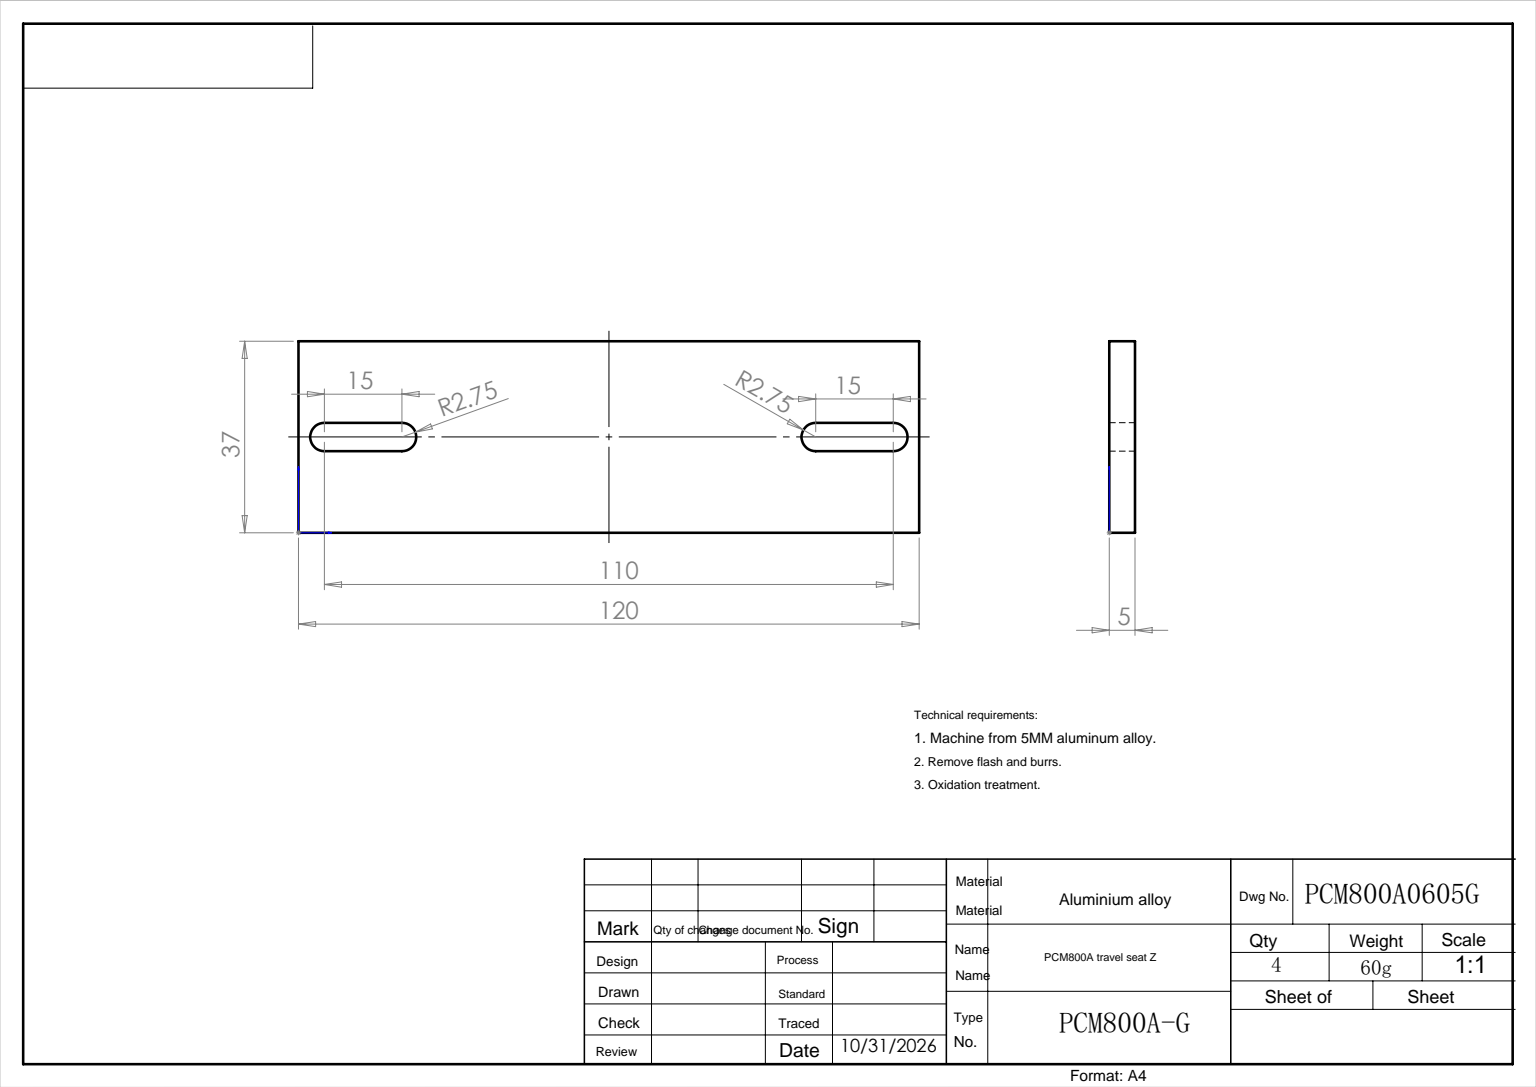
from build123d import *

# Parameters (mm, degrees)
SKETCH_1_W      = 120
SKETCH_1_H      = 37
EXTRUDE_1_DEPTH = 5


with BuildPart() as part:
    # 草图1 → 凸台-拉伸1 (new body)
    with BuildSketch(Plane.XY):
        with Locations((60, 18.5)):
            Rectangle(SKETCH_1_W, SKETCH_1_H)
        with BuildLine():
            Line((5, 21.25), (20, 21.25))
            ThreePointArc((20, 21.25), (22.75, 18.5), (20, 15.75))
            Line((20, 15.75), (5, 15.75))
            ThreePointArc((5, 15.75), (2.25, 18.5), (5, 21.25))
        make_face(mode=Mode.SUBTRACT)
        with BuildLine():
            Line((115, 15.75), (100, 15.75))
            ThreePointArc((100, 15.75), (97.25, 18.5), (100, 21.25))
            Line((100, 21.25), (115, 21.25))
            ThreePointArc((115, 21.25), (117.75, 18.5), (115, 15.75))
        make_face(mode=Mode.SUBTRACT)
    extrude(amount=EXTRUDE_1_DEPTH)


solid = part.part
